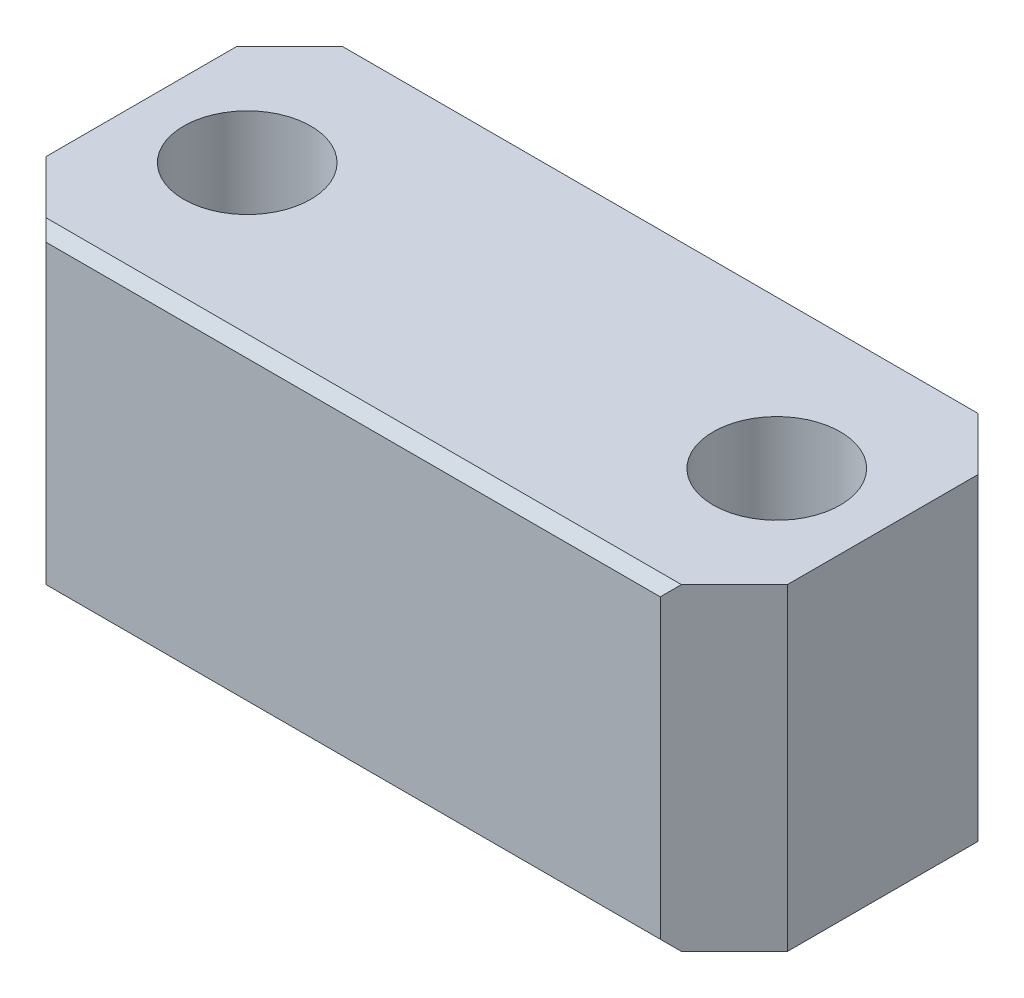
SolidWorks part; units mm, degrees
material "A6061"
ref_plane "Front Plane" through (0, 0, 0) normal (0, 0, 1) x (1, 0, 0)
ref_plane "Top Plane" through (0, 0, 0) normal (0, 1, 0) x (1, 0, 0)
ref_plane "Right Plane" through (0, 0, 0) normal (1, 0, 0) x (0, 0, -1)
sketch "Sketch1" plane through (0, 0, 0) normal (0, 1, 0) x (1, 0, 0)
  line L1 (-85.0733, 17.1348) -> (-50.0733, 17.1348)
  line L2 (-85.0733, 17.1348) -> (-85.0733, 2.1348)
  line L3 (-85.0733, 2.1348) -> (-50.0733, 2.1348)
  line L4 (-50.0733, 17.1348) -> (-50.0733, 2.1348)
  dimension "D1" = 35
  dimension "D2" = 15
extrude "Boss-Extrude1" add sketch "Sketch1" along normal blind 15
sketch "Sketch2" plane through (0, 15, 0) normal (0, 1, 0) x (1, 0, 0)
  line L0 (-50.0733, 2.1348) -> (-50.0733, 17.1348) construction
  circle A0 centre (-80.0733, 9.6348) radius 3
  circle A1 centre (-55.0733, 9.6348) radius 3
  dimension "D2" = 6
  dimension "D3" = 6
  dimension "D4" = 5
  dimension "D1" = 25
extrude "Cut-Extrude1" cut sketch "Sketch2" against normal blind 15.7
chamfer "Chamfer1" distance 3 angle 45 4 edges at (-50.0733, 7.5, -2.1348) (-50.0733, 7.5, -17.1348) (-85.0733, 7.5, -2.1348) (-85.0733, 7.5, -17.1348)
chamfer "Chamfer2" distance 0.5 angle 45 4 edges at (-67.5733, 0, -17.1348) (-67.5733, 0, -2.1348) (-67.5733, 15, -2.1348) (-67.5733, 15, -17.1348)
